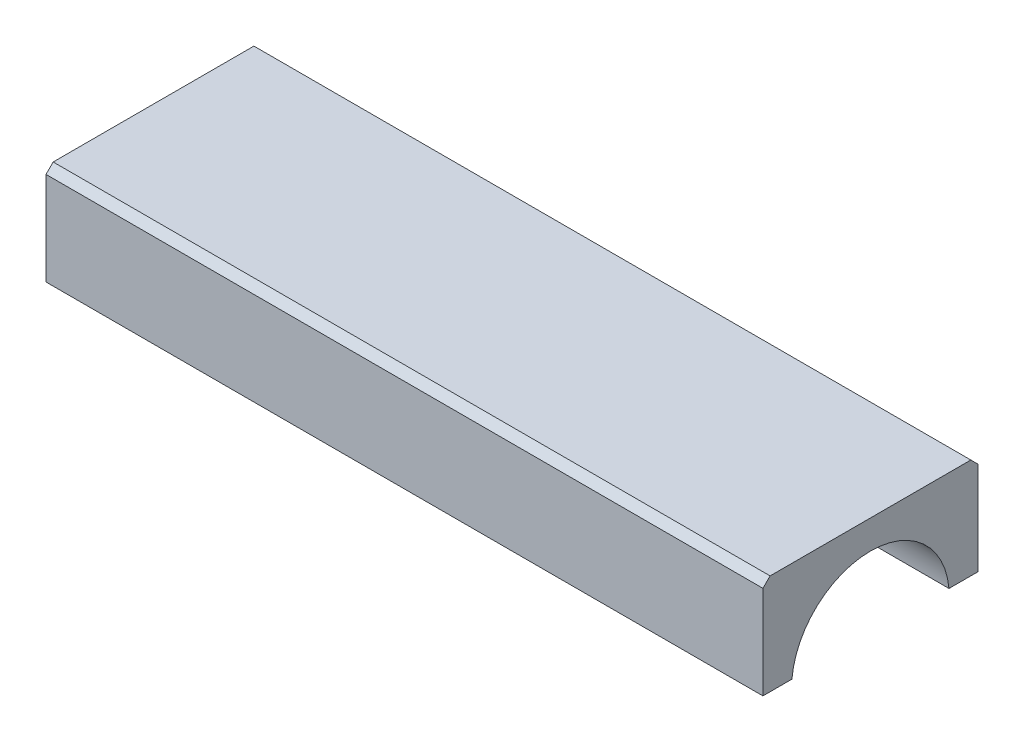
from build123d import *

# Parameters (mm, degrees)
SKETCH1_W           = 100
SKETCH1_H           = 14
BOSS_EXTRUDE1_DEPTH = 30
SKETCH2_R           = 11
CUT_EXTRUDE1_DEPTH  = 105.637469388
CHAMFER1_SIZE       = 1


with BuildPart() as part:
    # Sketch1 → Boss-Extrude1 (new body)
    with BuildSketch(Plane.XY):
        Rectangle(SKETCH1_W, SKETCH1_H)
    extrude(amount=BOSS_EXTRUDE1_DEPTH)

    # Sketch2 → Cut-Extrude1 (cut, through all)
    with BuildSketch(Plane.ZY.offset(50)):
        with Locations((15, -8)):
            Circle(SKETCH2_R)
    extrude(amount=-CUT_EXTRUDE1_DEPTH, mode=Mode.SUBTRACT)

    # Chamfer1
    chamfer1_edges = [part.edges().sort_by_distance(p)[0] for p in [
        (0, 7, 0),
        (0, 7, 30),
    ]]
    chamfer(chamfer1_edges, length=CHAMFER1_SIZE)


solid = part.part
